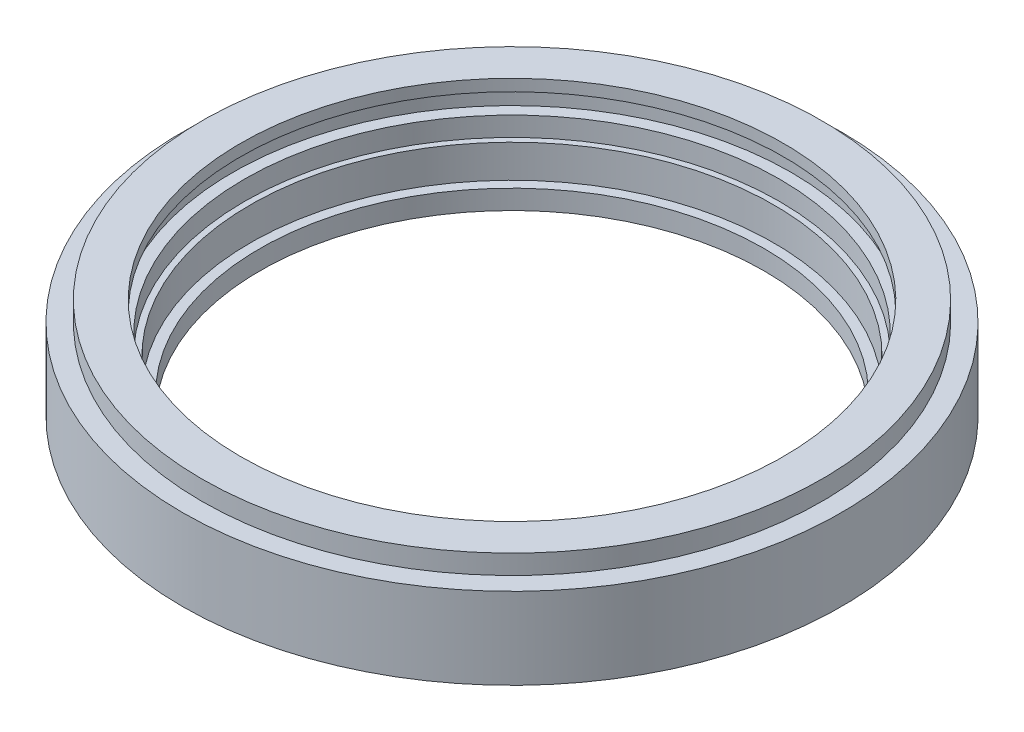
from build123d import *


with BuildPart() as part:
    # Sketch1 → Revolve1 (revolve)
    with BuildSketch(Plane.XY, mode=Mode.PRIVATE) as revolve1_sk:
        Polygon((70, 0), (80, 0), (80, -5), (85, -5), (85, -26), (65, -26), (65, -21), (67.5, -21), (67.5, -12.5), (69, -12.5), (69, -7.5), (72, -7.5), (72, -3), (70, -3), align=None)
    revolve(revolve1_sk.sketch.rotate(Axis((0, 0, 0), (0, -1, 0)), 90), axis=Axis((0, 0, 0), (0, -1, 0)))


solid = part.part
